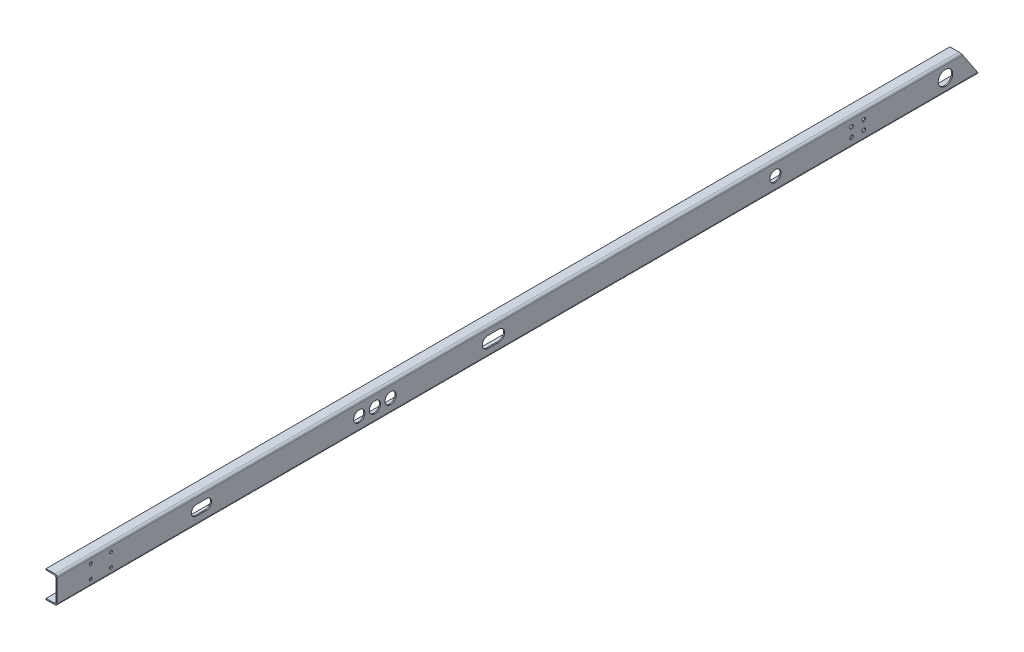
from build123d import *

# Parameters (mm, degrees)
EXTRUDE_1_DEPTH     = 4120
SKETCH_2_R          = 6.5
SKETCH_2_R_2        = 25
SKETCH_2_R_3        = 22.5
SKETCH_2_R_4        = 8
CUT_EXTRUDE_2_DEPTH = 10
CUT_EXTRUDE_3_DEPTH = 10
SKETCH_4_R          = 6.5
CUT_EXTRUDE_4_DEPTH = 10
SKETCH_5_W          = 22.746399217
SKETCH_5_H          = 81.53462818
SKETCH_5_R          = 6.5
EXTRUDE_2_DEPTH     = 5
SKETCH_6_R          = 32.5
CUT_EXTRUDE_5_DEPTH = 10
CUT_EXTRUDE_6_DEPTH = 63


with BuildPart() as part:
    # 草图1 → 凸台-拉伸1 (new body)
    with BuildSketch(Plane.XY):
        with BuildLine():
            Line((626.175555556, -48.428888889), (666.175555556, -48.428888889))
            ThreePointArc((666.175555556, -48.428888889), (673.246623367, -45.499956701), (676.175555556, -38.428888889))
            Line((676.175555556, -38.428888889), (676.175555556, 61.571111111))
            ThreePointArc((676.175555556, 61.571111111), (673.246623367, 68.642178923), (666.175555556, 71.571111111))
            Line((666.175555556, 71.571111111), (626.175555556, 71.571111111))
            Line((626.175555556, 71.571111111), (626.175555556, 66.571111111))
            Line((626.175555556, 66.571111111), (661.175555556, 66.571111111))
            ThreePointArc((661.175555556, 66.571111111), (668.246623367, 63.642178923), (671.175555556, 56.571111111))
            Line((671.175555556, 56.571111111), (671.175555556, -33.428888889))
            ThreePointArc((671.175555556, -33.428888889), (668.246623367, -40.499956701), (661.175555556, -43.428888889))
            Line((661.175555556, -43.428888889), (626.175555556, -43.428888889))
            Line((626.175555556, -43.428888889), (626.175555556, -48.428888889))
        make_face()
    extrude(amount=EXTRUDE_1_DEPTH)

    # 草图2 → 切除-拉伸2 (cut)
    with BuildSketch(Plane(origin=(676.175555556, 0, 0), x_dir=(0, 0, -1), z_dir=(1, 0, 0))):
        with Locations((-3985, -18.428888889)):
            Circle(SKETCH_2_R)
        with Locations((-3985, 41.571111111)):
            Circle(SKETCH_2_R)
        with Locations((-3895, 41.571111111)):
            Circle(SKETCH_2_R)
        with Locations((-3895, -18.428888889)):
            Circle(SKETCH_2_R)
        with Locations((-2770, 11.571111111)):
            Circle(SKETCH_2_R_2)
        with Locations((-2700, 11.571111111)):
            Circle(SKETCH_2_R_2)
        with Locations((-2630, 11.571111111)):
            Circle(SKETCH_2_R_2)
        with Locations((-150, 11.571111111)):
            Circle(SKETCH_2_R_3)
        with Locations((-570, 31.571111111)):
            Circle(SKETCH_2_R_4)
        with Locations((-515, 31.571111111)):
            Circle(SKETCH_2_R_4)
        with Locations((-570, -8.428888889)):
            Circle(SKETCH_2_R_4)
        with Locations((-515, -8.428888889)):
            Circle(SKETCH_2_R_4)
        with BuildLine():
            Line((-3497.5, 34.071111111), (-3452.5, 34.071111111))
            ThreePointArc((-3452.5, 34.071111111), (-3430, 11.571111111), (-3452.5, -10.928888889))
            Line((-3452.5, -10.928888889), (-3497.5, -10.928888889))
            ThreePointArc((-3497.5, -10.928888889), (-3520, 11.571111111), (-3497.5, 34.071111111))
        make_face()
        with BuildLine():
            Line((-2195, 36.571111111), (-2145, 36.571111111))
            ThreePointArc((-2145, 36.571111111), (-2120, 11.571111111), (-2145, -13.428888889))
            Line((-2145, -13.428888889), (-2195, -13.428888889))
            ThreePointArc((-2195, -13.428888889), (-2220, 11.571111111), (-2195, 36.571111111))
        make_face()
    extrude(amount=-CUT_EXTRUDE_2_DEPTH, mode=Mode.SUBTRACT)

    # 草图3 → 切除-拉伸3 (cut)
    with BuildSketch(Plane(origin=(676.175555556, 0, 0), x_dir=(0, 0, -1), z_dir=(1, 0, 0))):
        with BuildLine():
            ThreePointArc((-885, 11.571111111), (-892.32233047, 29.248780641), (-910, 36.571111111))
            Line((-910, 36.571111111), (-910, -13.428888889))
            ThreePointArc((-910, -13.428888889), (-892.32233047, -6.106558419), (-885, 11.571111111))
        make_face()
        with BuildLine():
            Line((-910, -13.428888889), (-910, 36.571111111))
            ThreePointArc((-910, 36.571111111), (-935, 11.571111111), (-910, -13.428888889))
        make_face()
    extrude(amount=-CUT_EXTRUDE_3_DEPTH, mode=Mode.SUBTRACT)

    # 草图4 → 切除-拉伸4 (cut)
    with BuildSketch(Plane(origin=(676.175555556, 0, 0), x_dir=(0, 0, -1), z_dir=(1, 0, 0))):
        with Locations((-3880, 41.571111111)):
            Circle(SKETCH_4_R)
        with Locations((-3970, 41.571111111)):
            Circle(SKETCH_4_R)
        with Locations((-3970, -18.428888889)):
            Circle(SKETCH_4_R)
        with Locations((-3880, -18.428888889)):
            Circle(SKETCH_4_R)
    extrude(amount=-CUT_EXTRUDE_4_DEPTH, mode=Mode.SUBTRACT)

    # 草图5 → 凸台-拉伸2 (add)
    # profile 1 of 6: a face of its own
    with BuildSketch(Plane(origin=(676.175555556, 0, 0), x_dir=(0, 0, -1), z_dir=(1, 0, 0))):
        with Locations((-3988.902277588, 11.372267682)):
            Rectangle(SKETCH_5_W, SKETCH_5_H)
        with Locations((-3985, 41.571111111)):
            Circle(SKETCH_5_R, mode=Mode.SUBTRACT)
        with Locations((-3985, -18.428888889)):
            Circle(SKETCH_5_R, mode=Mode.SUBTRACT)
    # profile 2 of 6: a face of its own
    with BuildSketch(Plane(origin=(676.175555556, 0, 0), x_dir=(0, 0, -1), z_dir=(1, 0, 0))):
        Polygon((-3887.411741686, 56.036728607), (-3911.283955206, 53.905280971), (-3903.726029575, -30.743486096), (-3887.411741686, -30.743486096), (-3887.411741686, -18.428888889), align=None)
        with Locations((-3895, -18.428888889)):
            Circle(SKETCH_5_R, mode=Mode.SUBTRACT)
        with Locations((-3895, 41.571111111)):
            Circle(SKETCH_5_R, mode=Mode.SUBTRACT)
    # profile 3 of 6: a face of its own
    with BuildSketch(Plane(origin=(676.175555556, 0, 0), x_dir=(0, 0, -1), z_dir=(1, 0, 0))):
        with Locations((-3985, 41.571111111)):
            Circle(SKETCH_5_R)
    # profile 4 of 6: a face of its own
    with BuildSketch(Plane(origin=(676.175555556, 0, 0), x_dir=(0, 0, -1), z_dir=(1, 0, 0))):
        with Locations((-3985, -18.428888889)):
            Circle(SKETCH_5_R)
    # profile 5 of 6: a face of its own
    with BuildSketch(Plane(origin=(676.175555556, 0, 0), x_dir=(0, 0, -1), z_dir=(1, 0, 0))):
        with Locations((-3895, -18.428888889)):
            Circle(SKETCH_5_R)
    # profile 6 of 6: a face of its own
    with BuildSketch(Plane(origin=(676.175555556, 0, 0), x_dir=(0, 0, -1), z_dir=(1, 0, 0))):
        with Locations((-3895, 41.571111111)):
            Circle(SKETCH_5_R)
    extrude(amount=-EXTRUDE_2_DEPTH)

    # 草图6 → 切除-拉伸5 (cut)
    with BuildSketch(Plane(origin=(676.175555556, 0, 0), x_dir=(0, 0, -1), z_dir=(1, 0, 0))):
        with Locations((-150, 11.571111111)):
            Circle(SKETCH_6_R)
    extrude(amount=-CUT_EXTRUDE_5_DEPTH, mode=Mode.SUBTRACT)

    # 草图7 → 切除-拉伸6 (cut)
    with BuildSketch(Plane(origin=(676.175555556, 0, 0), x_dir=(0, 0, -1), z_dir=(1, 0, 0))):
        Polygon((0, 71.571111111), (-80, 71.571111111), (0, -48.428888889), align=None)
    extrude(amount=-CUT_EXTRUDE_6_DEPTH, mode=Mode.SUBTRACT)


solid = part.part
